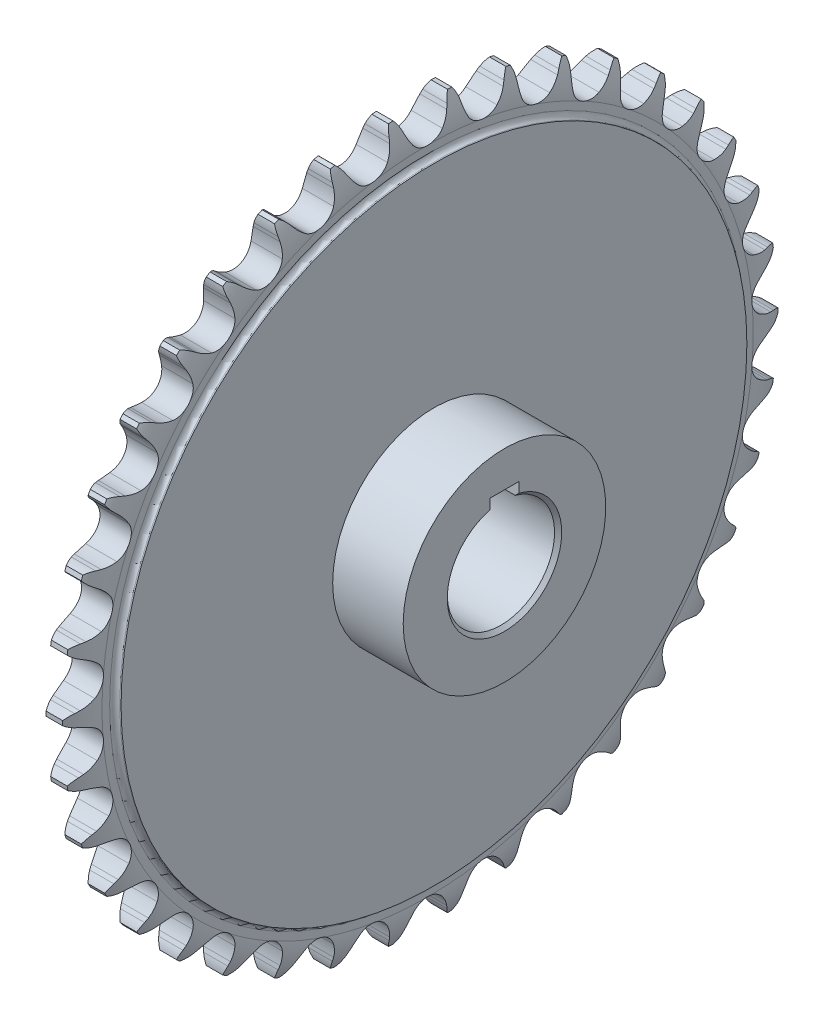
from build123d import *

# Parameters (mm, degrees)
CUT_EXTRUDE_1_DEPTH      = 6.140838417
PATTERN_CIRCULAR_1_COUNT = 38
SKETCH_3_W               = 19.718323166
SKETCH_3_H               = 13.322393537
SKETCH_4_W               = 8
SKETCH_4_H               = 3.843167657
CUT_EXTRUDE_2_DEPTH      = 145.79574468
CHAMFER_1_SIZE           = 1
CHAMFER_3_SIZE           = 1


with BuildPart() as part:
    # 草图1 → 旋转1 (revolve)
    with BuildSketch(Plane.XY, mode=Mode.PRIVATE) as revolve_1_sk:
        with BuildLine():
            Line((-6.140838417, 15), (-6.140838417, 87.5))
            Line((-6.140838417, 87.5), (-5.786870734, 87.5))
            ThreePointArc((-5.786870734, 87.5), (-4.785698937, 87.914698937), (-4.371, 88.915870734))
            Line((-4.371, 88.915870734), (-4.371, 91.039676834))
            ThreePointArc((-4.371, 91.039676834), (-4.002065081, 95.672527396), (-2.30725, 100))
            Line((-2.30725, 100), (2.30725, 100))
            ThreePointArc((2.30725, 100), (4.002065081, 95.672527396), (4.371, 91.039676834))
            Line((4.371, 91.039676834), (4.371, 88.915870734))
            ThreePointArc((4.371, 88.915870734), (4.785698937, 87.914698937), (5.786870734, 87.5))
            Line((5.786870734, 87.5), (6.140838417, 87.5))
            Line((6.140838417, 87.5), (6.140838417, 15))
            Line((6.140838417, 15), (-6.140838417, 15))
        make_face()
    revolve(revolve_1_sk.sketch.rotate(Axis((-7.9375, 0, 0), (1, 0, 0)), 90), axis=Axis((-7.9375, 0, 0), (1, 0, 0)))

    # 草图2 → 切除-拉伸1 (cut, symmetric)
    with BuildSketch(Plane(origin=(0, 0, 0), x_dir=(0, 0, -1), z_dir=(1, 0, 0))):
        with BuildLine():
            Line((5.951053701, 96.408740014), (6.354520938, 97.514096797))
            ThreePointArc((6.354520938, 97.514096797), (6.894671031, 98.667537105), (7.628391875, 99.708613657))
            ThreePointArc((7.628391875, 99.708613657), (0, 100), (-7.628391875, 99.708613657))
            ThreePointArc((-7.628391875, 99.708613657), (-6.894671031, 98.667537105), (-6.354520938, 97.514096797))
            Line((-6.354520938, 97.514096797), (-5.951053701, 96.408740014))
            ThreePointArc((-5.951053701, 96.408740014), (-5.166916335, 94.662668482), (-4.139974354, 93.047420089))
            ThreePointArc((-4.139974354, 93.047420089), (0, 90.964276834), (4.139974354, 93.047420089))
            ThreePointArc((4.139974354, 93.047420089), (5.166916335, 94.662668482), (5.951053701, 96.408740014))
        make_face()
    cut_extrude_1 = extrude(amount=CUT_EXTRUDE_1_DEPTH, both=True, mode=Mode.SUBTRACT)

    # 阵列(圆周)1: 切除-拉伸1 ×38 about axis
    pattern_circular_1_axis = Axis((0, 0, 0), (1, 0, 0))
    for i in range(1, PATTERN_CIRCULAR_1_COUNT):
        add(cut_extrude_1.rotate(pattern_circular_1_axis, i * 360 / PATTERN_CIRCULAR_1_COUNT), mode=Mode.SUBTRACT)

    # 草图3 → 旋转2 (revolve)
    with BuildSketch(Plane.XY, mode=Mode.PRIVATE) as revolve_2_sk:
        with Locations((16, 21.661196769)):
            Rectangle(SKETCH_3_W, SKETCH_3_H)
    revolve(revolve_2_sk.sketch.rotate(Axis((0, 0, 0), (1, 0, 0)), 90), axis=Axis((0, 0, 0), (1, 0, 0)))

    # 草图4 → 切除-拉伸2 (cut, through all)
    with BuildSketch(Plane.ZY.offset(6.140838417)):
        with Locations((0, 16.378416124)):
            Rectangle(SKETCH_4_W, SKETCH_4_H)
    extrude(amount=-CUT_EXTRUDE_2_DEPTH, mode=Mode.SUBTRACT)

    # 倒角1
    chamfer_1_edges = [part.edges().sort_by_distance(p)[0] for p in [
        (-6.140838417, -15, 0),
    ]]
    chamfer(chamfer_1_edges, length=CHAMFER_1_SIZE)

    # 倒角3
    chamfer_3_edges = [part.edges().sort_by_distance(p)[0] for p in [
        (25.859161583, -15, 0),
    ]]
    chamfer(chamfer_3_edges, length=CHAMFER_3_SIZE)


solid = part.part
